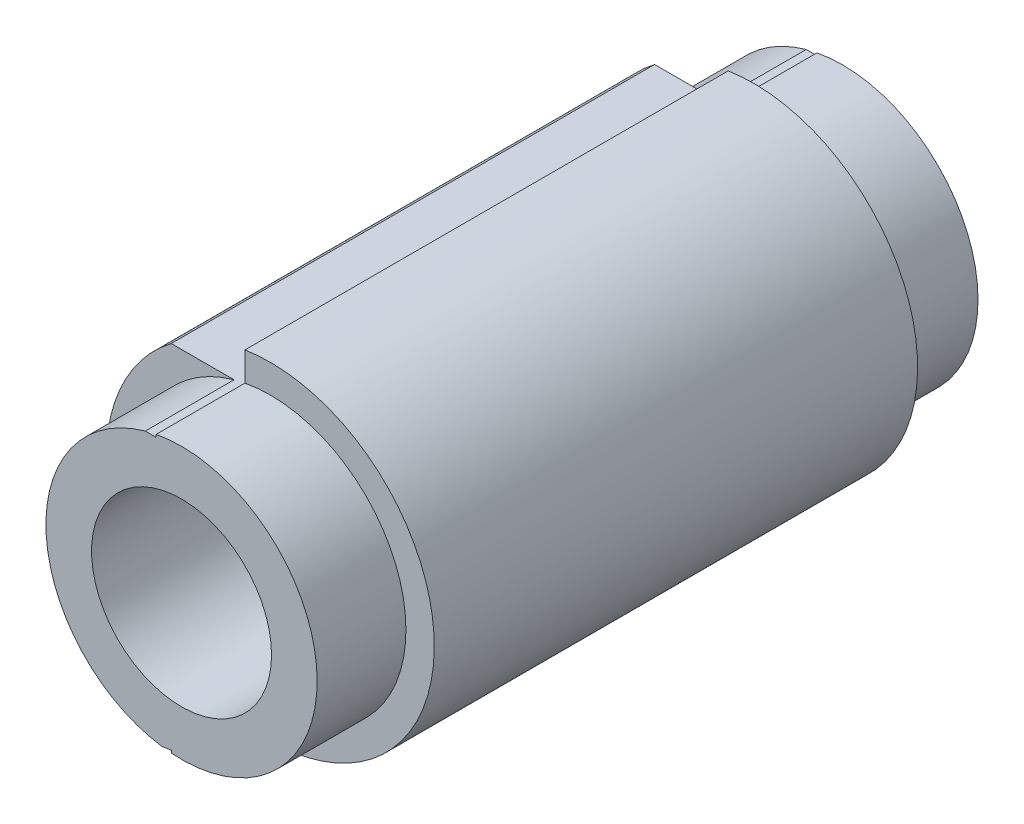
from build123d import *

# Parameters (mm, degrees)
SKETCH1_R           = 36.5
BOSS_EXTRUDE1_DEPTH = 268
SKETCH2_R           = 70
SKETCH2_R_2         = 55
CUT_EXTRUDE1_DEPTH  = 36
CUT_EXTRUDE2_START  = -36
SKETCH3_R           = 70
SKETCH3_R_2         = 55
CUT_EXTRUDE2_DEPTH  = 36


with BuildPart() as part:
    # Sketch1 → Boss-Extrude1 (new body)
    with BuildSketch(Plane.XY):
        with BuildLine():
            Line((-40.165283517, 53), (-10.3, 53))
            Line((-10.3, 53), (-10.3, 65.697488536))
            ThreePointArc((-10.3, 65.697488536), (66.373170096, 4.105154246), (-2.125739686, -66.466015608))
            Line((-2.125739686, -66.466015608), (-4.128100838, -53.823604848))
            Line((-4.128100838, -53.823604848), (-32.079680877, -58.250700209))
            ThreePointArc((-32.079680877, -58.250700209), (-66.325057816, -4.820446627), (-40.165283517, 53))
        make_face()
        Circle(SKETCH1_R, mode=Mode.SUBTRACT)
    extrude(amount=BOSS_EXTRUDE1_DEPTH)

    # Sketch2 → Cut-Extrude1 (cut)
    with BuildSketch(Plane.XY.offset(268)):
        Circle(SKETCH2_R)
        Circle(SKETCH2_R_2, mode=Mode.SUBTRACT)
    extrude(amount=-CUT_EXTRUDE1_DEPTH, mode=Mode.SUBTRACT)

    # Sketch3 → Cut-Extrude2 (cut)
    with BuildSketch(Plane(origin=(0, 0, 0), x_dir=(-1, 0, 0), z_dir=(0, 0, -1)).offset(CUT_EXTRUDE2_START)):
        Circle(SKETCH3_R)
        Circle(SKETCH3_R_2, mode=Mode.SUBTRACT)
    extrude(amount=CUT_EXTRUDE2_DEPTH, mode=Mode.SUBTRACT)


solid = part.part
